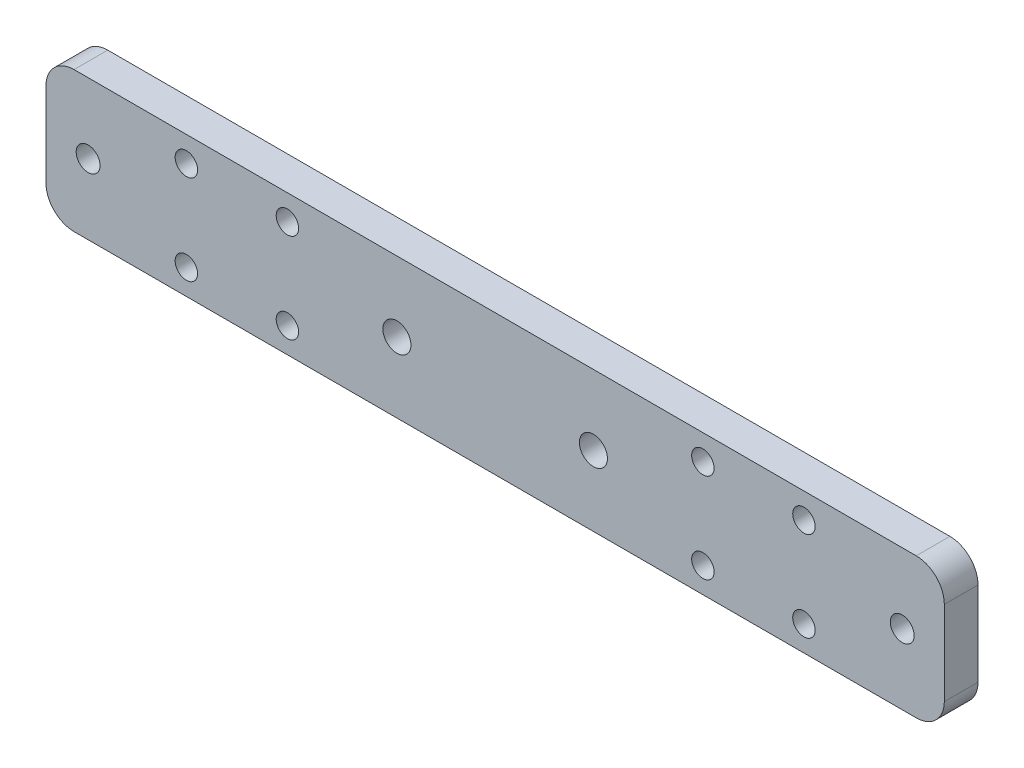
from build123d import *

# Parameters (mm, degrees)
SKETCH1_W              = 320
SKETCH1_H              = 50
SKETCH1_R              = 4
SKETCH1_R_2            = 5
BOSS_EXTRUDE1_DEPTH    = 12
M10_TAPPED_HOLE1_D     = 8.5
M10_TAPPED_HOLE1_DEPTH = 24.5
M10_TAPPED_HOLE1_TIP   = 2.553657631
FILLET1_R              = 10


with BuildPart() as part:
    # Sketch1 → Boss-Extrude1 (new body)
    with BuildSketch(Plane.XY):
        with Locations((160, 25)):
            Rectangle(SKETCH1_W, SKETCH1_H)
        with Locations((50, 41)):
            Circle(SKETCH1_R, mode=Mode.SUBTRACT)
        with Locations((86, 41)):
            Circle(SKETCH1_R, mode=Mode.SUBTRACT)
        with Locations(Location((86, 9, 0), (0, 0, 180))):
            Circle(SKETCH1_R, mode=Mode.SUBTRACT)
        with Locations(Location((50, 9, 0), (0, 0, 180))):
            Circle(SKETCH1_R, mode=Mode.SUBTRACT)
        with Locations((270, 9)):
            Circle(SKETCH1_R, mode=Mode.SUBTRACT)
        with Locations((234, 9)):
            Circle(SKETCH1_R, mode=Mode.SUBTRACT)
        with Locations(Location((234, 41, 0), (0, 0, 180))):
            Circle(SKETCH1_R, mode=Mode.SUBTRACT)
        with Locations(Location((270, 41, 0), (0, 0, 180))):
            Circle(SKETCH1_R, mode=Mode.SUBTRACT)
        with Locations((125, 25)):
            Circle(SKETCH1_R_2, mode=Mode.SUBTRACT)
        with Locations((195, 25)):
            Circle(SKETCH1_R_2, mode=Mode.SUBTRACT)
    extrude(amount=BOSS_EXTRUDE1_DEPTH)

    # M10 Tapped Hole1
    with Locations(Plane.XY.offset(12)):
        with Locations((15, 25), (305, 25)):
            Hole(M10_TAPPED_HOLE1_D / 2, depth=M10_TAPPED_HOLE1_DEPTH)
            with Locations((0, 0, -(M10_TAPPED_HOLE1_DEPTH + M10_TAPPED_HOLE1_TIP / 2))):  # 118° drill point
                Cone(0, M10_TAPPED_HOLE1_D / 2, M10_TAPPED_HOLE1_TIP, mode=Mode.SUBTRACT)

    # Fillet1
    fillet1_edges = [part.edges().sort_by_distance(p)[0] for p in [
        (320, 0, 6),
        (0, 0, 6),
        (0, 50, 6),
        (320, 50, 6),
    ]]
    fillet(fillet1_edges, radius=FILLET1_R)


solid = part.part
